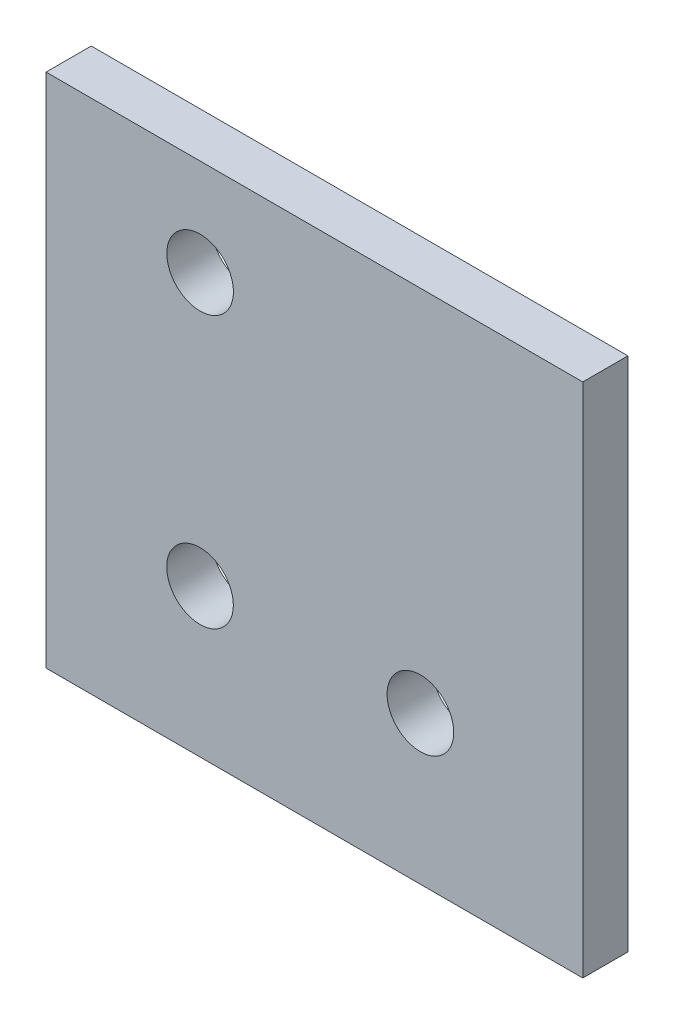
SolidWorks part; units mm, degrees
material "普通碳钢"
ref_plane "Front Plane" through (0, 0, 0) normal (0, 0, 1) x (1, 0, 0)
ref_plane "Top Plane" through (0, 0, 0) normal (0, 1, 0) x (1, 0, 0)
ref_plane "Right Plane" through (0, 0, 0) normal (1, 0, 0) x (0, 0, -1)
sketch "Sketch1" plane through (0, 0, 0) normal (0, 0, 1) x (1, 0, 0)
  line L0 (87.2467, -34.102) -> (-93.0764, -34.102) construction
  line L1 (-83.175, 80) -> (83.175, 80)
  line L2 (-83.175, 80) -> (-83.175, -80)
  line L3 (-83.175, -80) -> (83.175, -80)
  line L4 (83.175, 80) -> (83.175, -80)
  line L5 (-83.175, 80) -> (83.175, -80) construction
  line L6 (-83.175, -80) -> (83.175, 80) construction
  line L7 (-35.423, 83.2507) -> (-35.423, -98.5225) construction
  line L8 (-89.256, 50.048) -> (-0.5935, 50.048) construction
  line L9 (32.852, -24.9545) -> (32.852, -98.5225) construction
  circle A0 centre (-35.423, 50.048) radius 10.325
  circle A1 centre (-35.4554, -34.102) radius 10.325
  circle A2 centre (32.852, -34.102) radius 10.325
  point P0 (0, 0)
  dimension "D7" = 20.65
  dimension "D1" = 166.35
  dimension "D2" = 160
  dimension "D3" = 47.752
  dimension "D4" = 45.898
  dimension "D5" = 84.15
  dimension "D6" = 68.275
extrude "Boss-Extrude1" add sketch "Sketch1" along normal blind 14
